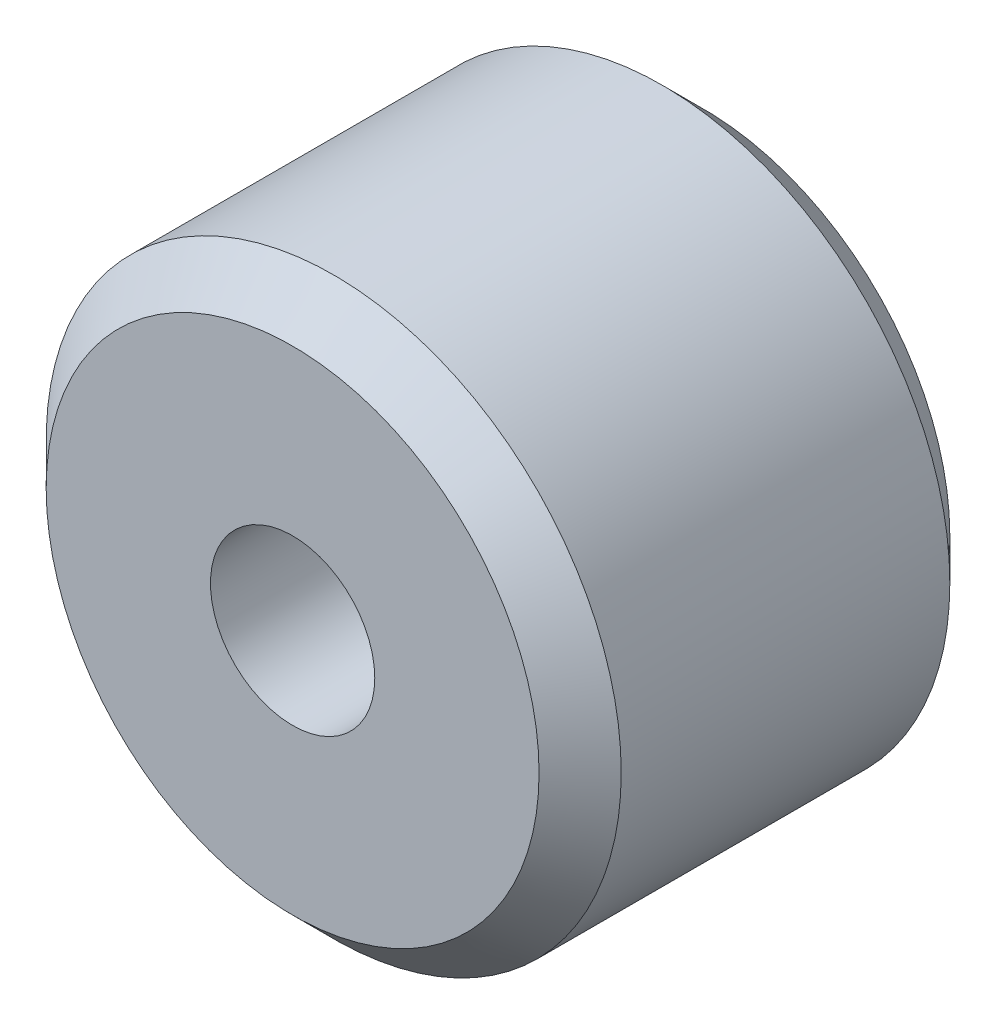
SolidWorks part; units mm, degrees
ref_plane "Front Plane" through (0, 0, 0) normal (0, 0, 1) x (1, 0, 0)
ref_plane "Top Plane" through (0, 0, 0) normal (0, 1, 0) x (1, 0, 0)
ref_plane "Right Plane" through (0, 0, 0) normal (1, 0, 0) x (0, 0, -1)
other "Configuration Table"
sketch "Sketch1" plane through (0, 0, 0) normal (0, 0, 1) x (1, 0, 0)
  circle A0 centre (0, 0) radius 3.5
  dimension "D1" = 7
extrude "Boss-Extrude1" add sketch "Sketch1" along normal blind 5
sketch "Sketch2" plane through (0, 0, 5) normal (0, 0, 1) x (1, 0, 0)
  circle A0 centre (0, 0) radius 1
  dimension "D1" = 2
extrude "Cut-Extrude1" cut sketch "Sketch2" against normal blind 11
chamfer "Chamfer1" distance 0.5 angle 45 2 edges at (3.5, 0, 0) (3.5, 0, 5)
